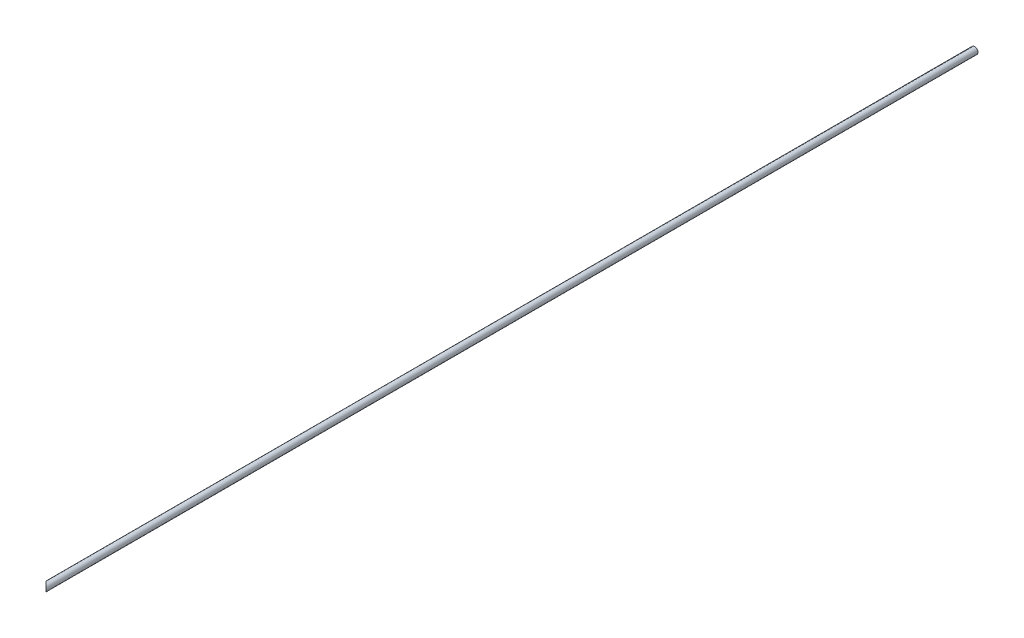
from build123d import *

# Parameters (mm, degrees)
SKETCH1_R               = 3
BOSS_EXTRUDE1_DEPTH     = 832.8
CUT_EXTRUDE1_DEPTH      = 833.810806846
CUT_EXTRUDE1_DEPTH_BACK = 833.810806846


with BuildPart() as part:
    # Sketch1 → Boss-Extrude1 (new body)
    with BuildSketch(Plane.XY):
        Circle(SKETCH1_R)
    extrude(amount=BOSS_EXTRUDE1_DEPTH)

    # Sketch2 → Cut-Extrude1 (cut, two sides: drawn at the far end of the back side and taken through both)
    with BuildSketch(Plane(origin=(0, 0, 0), x_dir=(1, 0, 0), z_dir=(0, 1, 0)).offset(-CUT_EXTRUDE1_DEPTH_BACK)):
        Polygon((3, -832.8), (-3, -826.8), (-3, -832.8), align=None)
    extrude(amount=CUT_EXTRUDE1_DEPTH + CUT_EXTRUDE1_DEPTH_BACK, mode=Mode.SUBTRACT)


solid = part.part
